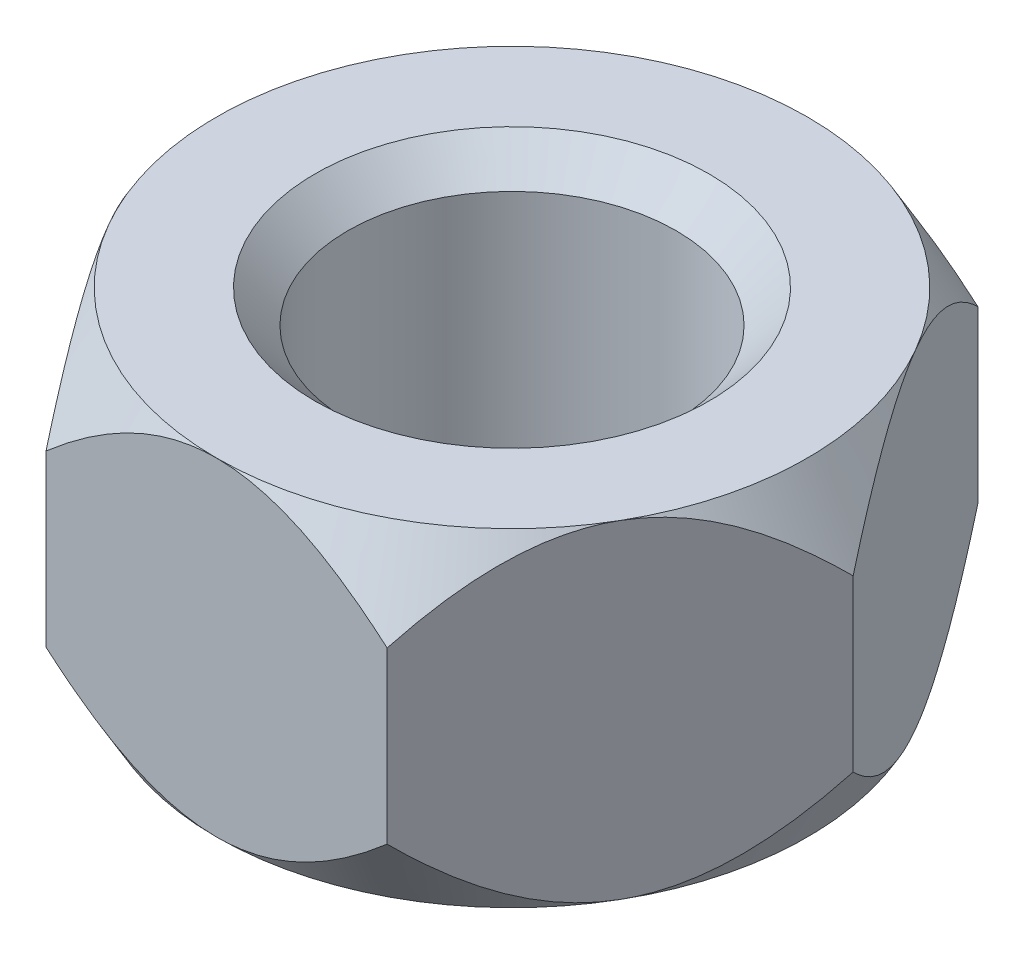
from build123d import *

# Parameters (mm, degrees)
BOSS_EXTRUDE1_DEPTH = 5
SKETCH2_R           = 2.5
CUT_EXTRUDE1_DEPTH  = 5
SKETCH3_OUTSIDE_W   = 21.092
SKETCH3_OUTSIDE_H   = 19.7
SKETCH3_OUTSIDE_R   = 4.5
CUT_EXTRUDE2_DEPTH  = 5
CUT_EXTRUDE2_DRAFT  = -30
SKETCH4_OUTSIDE_W   = 21.092
SKETCH4_OUTSIDE_H   = 19.7
SKETCH4_OUTSIDE_R   = 4.5
CUT_EXTRUDE3_DEPTH  = 5
CUT_EXTRUDE3_DRAFT  = -30
CHAMFER1_SIZE       = 0.5
CHAMFER2_SIZE       = 0.5


with BuildPart() as part:
    # Sketch1 → Boss-Extrude1 (new body)
    with BuildSketch(Plane(origin=(0, 0, 0), x_dir=(1, 0, 0), z_dir=(0, 1, 0))):
        Polygon((2.598076211, 4.5), (-2.598076211, 4.5), (-5.196152423, 0), (-2.598076211, -4.5), (2.598076211, -4.5), (5.196152423, 0), align=None)
    extrude(amount=BOSS_EXTRUDE1_DEPTH)

    # Sketch2 → Cut-Extrude1 (cut)
    with BuildSketch(Plane(origin=(0, 5, 0), x_dir=(1, 0, 0), z_dir=(0, 1, 0))):
        with Locations(Location((0, 0, 0), (0, 0, 270))):
            Circle(SKETCH2_R)
    extrude(amount=-CUT_EXTRUDE1_DEPTH, mode=Mode.SUBTRACT)


with BuildPart() as cut_extrude2_tool:
    # Sketch3 outside → Cut-Extrude2 (with draft: the straight prism first)
    with BuildSketch(Plane(origin=(0, 5, 0), x_dir=(1, 0, 0), z_dir=(0, 1, 0))):
        Rectangle(SKETCH3_OUTSIDE_W, SKETCH3_OUTSIDE_H)
        Circle(SKETCH3_OUTSIDE_R, mode=Mode.SUBTRACT)
    extrude(amount=-CUT_EXTRUDE2_DEPTH)
    # Cut-Extrude2: the draft: its side faces are tilted about the plane it starts from
    cut_extrude2_sides = [cut_extrude2_tool.faces().sort_by_distance(p)[0] for p in [
        (0, 2.5, 9.85),
        (10.546, 2.5, 0),
        (0, 2.5, -9.85),
        (-10.546, 2.5, 0),
        (-4.5, 2.5, 0),
    ]]
    draft(cut_extrude2_sides, Plane(origin=(0, 5, 0), x_dir=(1, 0, 0), z_dir=(0, 1, 0)), CUT_EXTRUDE2_DRAFT)


with BuildPart() as part_1:
    add(part.part)

    # Cut-Extrude2: cut by cut_extrude2_tool
    add(cut_extrude2_tool.part, mode=Mode.SUBTRACT)


with BuildPart() as cut_extrude3_tool:
    # Sketch4 outside → Cut-Extrude3 (with draft: the straight prism first)
    with BuildSketch(Plane.XZ):
        Rectangle(SKETCH4_OUTSIDE_W, SKETCH4_OUTSIDE_H)
        Circle(SKETCH4_OUTSIDE_R, mode=Mode.SUBTRACT)
    extrude(amount=-CUT_EXTRUDE3_DEPTH)
    # Cut-Extrude3: the draft: its side faces are tilted about the plane it starts from
    cut_extrude3_sides = [cut_extrude3_tool.faces().sort_by_distance(p)[0] for p in [
        (0, 2.5, -9.85),
        (10.546, 2.5, 0),
        (0, 2.5, 9.85),
        (-10.546, 2.5, 0),
        (-4.5, 2.5, 0),
    ]]
    draft(cut_extrude3_sides, Plane.XZ, CUT_EXTRUDE3_DRAFT)


with BuildPart() as part_2:
    add(part_1.part)

    # Cut-Extrude3: cut by cut_extrude3_tool
    add(cut_extrude3_tool.part, mode=Mode.SUBTRACT)

    # Chamfer1
    chamfer1_edges = [part_2.edges().sort_by_distance(p)[0] for p in [
        (0, 5, -2.5),
    ]]
    chamfer(chamfer1_edges, length=CHAMFER1_SIZE)

    # Chamfer2
    chamfer2_edges = [part_2.edges().sort_by_distance(p)[0] for p in [
        (0, 0, -2.5),
    ]]
    chamfer(chamfer2_edges, length=CHAMFER2_SIZE)


solid = part_2.part
